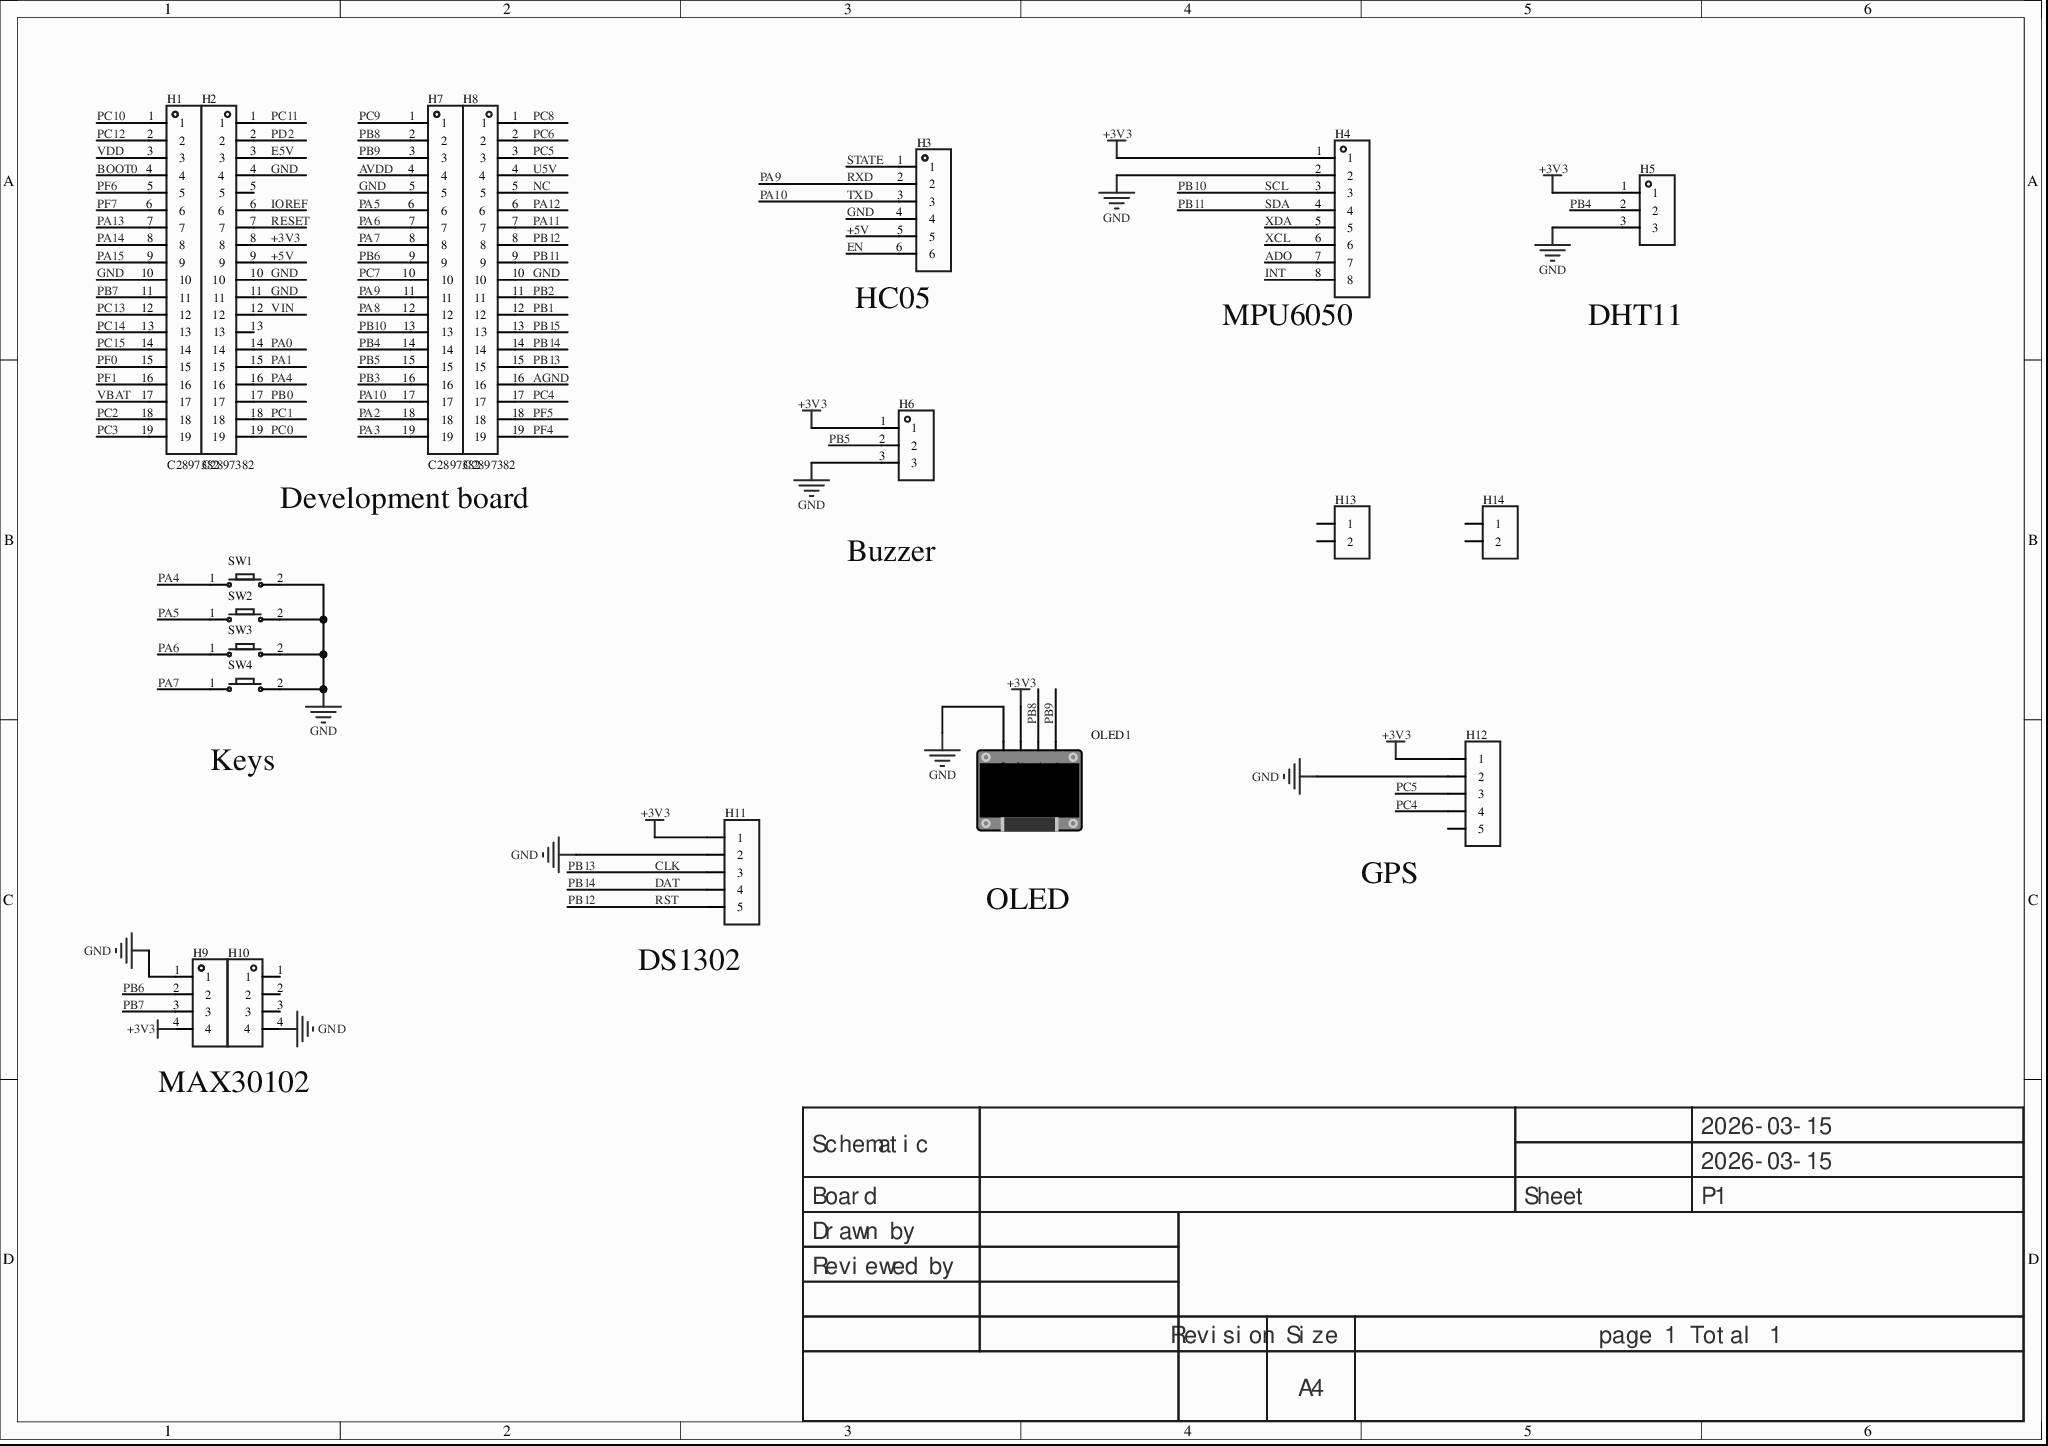
[diagram p0: MISC82907-3.schdoc]
# Altium project MISC82907-2.PrjPcb
1 sheet, 19 parts. Net scope: global (net labels, ports and power ports of the same name join across sheets).
Board file: MISC82907.pcbdoc

## Sheet MISC82907-3.schdoc
size 297 x 209 mm; Version: V1.0; @Project Name: MISC82907; @Update Date: 2026-03-15; @Create Date: 2026-03-15; @Board Name: MISC82907; @Create Time: 16:08:49; @Page Count: 1; @Page No: 1; @Schematic Name: MISC82907; @Update Time: 16:08:49; Size: A4

### Parts
H1  C2897382  [HDR-TH_19P-P2.54-V-F]
H2  C2897382  [HDR-TH_19P-P2.54-V-F]
H3  (no value)  [HDR-TH_6P-P2.54-V-F]
H4  (no value)  [HDR-TH_8P-P2.54-V-F-1]
H5  (no value)  [HDR-TH_3P-P2.54-V-F]
H6  (no value)  [HDR-TH_3P-P2.54-V-F]
H7  C2897382  [HDR-TH_19P-P2.54-V-F]
H8  C2897382  [HDR-TH_19P-P2.54-V-F]
H9  (no value)  [HDR-TH_4P-P2.54-V-F]
H10  (no value)  [HDR-TH_4P-P2.54-V-F]
H11  (no value)  [HDR-TH_5P-P2.54-V-F]
H12  (no value)  [HDR-TH_5P-P2.54-V-F]
H13  (no value)  [HDR-TH_2P-P2.54-V-F]
H14  (no value)  [HDR-TH_2P-P2.54-V-F]
OLED1  (no value)  [0.96OLED_4P]
SW1  (no value)  [Key_SMD_3.6x6.1x2.5]
SW2  (no value)  [Key_SMD_3.6x6.1x2.5]
SW3  (no value)  [Key_SMD_3.6x6.1x2.5]
SW4  (no value)  [Key_SMD_3.6x6.1x2.5]

### Nets
+3V3: H2.8 H4.1 H5.1 H6.1 H9.4 H11.1 H12.1 OLED1.2(VCC)
GND: H1.10 H2.4 H2.10 H2.11 H3.4 H4.2 H5.3 H6.3 H7.5 H8.10 H9.1 H10.4 H11.2 H12.2 OLED1.1(GND) SW1.2 SW2.2 SW3.2 SW4.2
+5V: H2.9 H3.5
ADO: H4.7
AGND: H8.16
AVDD: H7.4
BOOT0: H1.4
CLK: H8.15 H11.3  [also labelled PB13]
DAT: H8.14 H11.4  [also labelled PB14]
E5V: H2.3
EN: H3.6
INT: H4.8
IOREF: H2.6
NC: H8.5
PA0: H2.14
PA1: H2.15
PA2: H7.18
PA3: H7.19
PA4: H2.16 SW1.1
PA5: H7.6 SW2.1
PA6: H7.7 SW3.1
PA7: H7.8 SW4.1
PA8: H7.12
PA9: H3.2 H7.11  [also labelled RXD]
PA10: H3.3 H7.17  [also labelled TXD]
PA11: H8.7
PA12: H8.6
PA13: H1.7
PA14: H1.8
PA15: H1.9
PB0: H2.17
PB1: H8.12
PB2: H8.11
PB3: H7.16
PB4: H5.2 H7.14
PB5: H6.2 H7.15
PB6: H7.9 H9.2
PB7: H1.11 H9.3
PB8: H7.2 OLED1.3(SCL)
PB9: H7.3 OLED1.4(SDA)
PB10: H4.3 H7.13  [also labelled SCL]
PB11: H4.4 H8.9  [also labelled SDA]
PB12: H8.8 H11.5  [also labelled RST]
PB15: H8.13
PC0: H2.19
PC1: H2.18
PC2: H1.18
PC3: H1.19
PC4: H8.17 H12.4
PC5: H8.3 H12.3
PC6: H8.2
PC7: H7.10
PC8: H8.1
PC9: H7.1
PC10: H1.1
PC11: H2.1
PC12: H1.2
PC13: H1.12
PC14: H1.13
PC15: H1.14
PD2: H2.2
PF0: H1.15
PF1: H1.16
PF4: H8.19
PF5: H8.18
PF6: H1.5
PF7: H1.6
RESET: H2.7
STATE: H3.1
U5V: H8.4
VBAT: H1.17
VDD: H1.3
VIN: H2.12
XCL: H4.6
XDA: H4.5

Not connected (* = marked no-connect by the designer): H2 5 13; H10 1 2 3; H12 5; H13 1 2; H14 1 2

### Notes on the sheet
- (near H3) HC05
- (near H4) MPU6050
- DHT11
- Development board
- Buzzer
- (near SW4) Keys
- OLED
- (near H12) GPS
- (near H11) DS1302
- MAX30102
- 2026-03-15
- Schematic
- Board
- Sheet
- P1
- Drawn by
- Reviewed by
- Revision
- Size
- A4
- page 1 Total 1

### Library data of the parts
H1 H2 H7 H8 = HDR-F_2.54_1x19P: ConvertToPcb: yes; ModelId: 131ee080550a465daf9368d356f53fe90819f05c4eef4c71ace90d822a990e87; ModelName: HDR-TH_19P-P2.54-F-LI-1X19P; ModelTransform: 1919.68128,95.6691,0,0,0,0,0,0,-125.984; Symbol: HDR-F_2.54_1x19P; Device: HDR-F_2.54_1x19P; AddInBom: yes; Supplier Footprint: 插件; ManufacturerPart: C2897382; FootprintName: HDR-TH_19P-P2.54-V-F
H3 = HDR-F_2.54_1x6P: Symbol: Header-Female-2.54_1x6; ConvertToPcb: yes; ModelId: 0f5bcf94dcda47d085f24cdca1696fe90819f05c4eef4c71ace90d822a990e87; ModelTransform: 619.684,94.488,0,0,0,0,0,0,-125.984; Device: HDR-F_2.54_1x6P; AddInBom: yes; SupplierPart: C40877; Supplier Footprint: 插件; FootprintName: HDR-TH_6P-P2.54-V-F; ModelName: HDR-TH_6P-P2.54-V-F
H4 = HDR-F_2.54_1x8P: Symbol: Header-Female-2.54_1x8; AddInBom: yes; ModelId: 0f7e4d9227ef4fa08d5469c22cc70cdb0819f05c4eef4c71ace90d822a990e87; ModelName: HDR-F-2.54_1x8; ModelTransform: 799.99844,100,0,0,0,0,0,0,-118.11; Device: HDR-F_2.54_1x8P; ConvertToPcb: yes; FootprintName: HDR-TH_8P-P2.54-V-F-1; SupplierPart: C27438; Supplier Footprint: 插件
H5 H6 = HDR-F_2.54_1x3P: Symbol: PM254V-11-03-H85; ConvertToPcb: yes; ModelId: f3b3cc5aae9641bf9e56fc160cef875b0819f05c4eef4c71ace90d822a990e87; ModelName: HDR2.54-F-LI-1X3P; ModelTransform: 299.9994,100,0,0,0,0,0,0,-118.11; Device: HDR-F_2.54_1x3P; AddInBom: yes; SupplierPart: C541850; Supplier Footprint: 插件; FootprintName: HDR-TH_3P-P2.54-V-F
H9 H10 = HDR-F_2.54_1x4P: Symbol: 2.54-1*4P female; ConvertToPcb: yes; ModelId: d187812051054f85879fcaa51a310d8e0819f05c4eef4c71ace90d822a990e87; ModelTransform: 419.6842,98.464,0,0,0,0,0,0,-118.11; Device: HDR-F_2.54_1x4P; AddInBom: yes; SupplierPart: C2718488; Supplier Footprint: 插件; FootprintName: HDR-TH_4P-P2.54-V-F; ModelName: HDR-TH_4P-P2.54-V-F
H11 = HDR-F_2.54_1x5P: Symbol: Header-Female-2.54_1x5; ConvertToPcb: yes; ModelId: f49cb6116a3d45e5a64915bf3e00773f0819f05c4eef4c71ace90d822a990e87; ModelTransform: 519.684,98.464,0,0,0,0,0,0,-124.016; Device: HDR-F_2.54_1x5P; AddInBom: yes; SupplierPart: C50950; Supplier Footprint: 插件; FootprintName: HDR-TH_5P-P2.54-V-F; ModelName: HDR-TH_5P-P2.54-V-F
H12 = HDR-F_2.54_1x5P: Symbol: Header-Female-2.54_1x5; 3D Model: f49cb6116a3d45e5a64915bf3e00773f0819f05c4eef4c71ace90d822a990e87; 3D Model Transform: 519.684,98.464,0,0,0,0,0,0,-124.016; ConvertToPcb: yes; Device: HDR-F_2.54_1x5P; Supplier Part: C50950; Supplier Footprint: 插件; AddInBom: yes; FootprintName: HDR-TH_5P-P2.54-V-F; ModelName: HDR-TH_5P-P2.54-V-F
H13 H14 = HDR-F_2.54_1x2P: Symbol: Header-Female-2.54_1x2; ConvertToPcb: yes; ModelId: a9450ef445564560a104363b9aacde4e0819f05c4eef4c71ace90d822a990e87; ModelName: HDR-TH_2P-P2.54-F-LI-1X2P; ModelTransform: 215.7476,98.425,0,0,0,0,0,0,-129.921; Device: HDR-F_2.54_1x2P; AddInBom: yes; SupplierPart: C49661; Supplier Footprint: 插件; FootprintName: HDR-TH_2P-P2.54-V-F
OLED1 = 0.96OLED模块_4P: Symbol: 0.96OLED module_4P; ConvertToPcb: yes; ModelId: 79c000fdb68d45a296c2e9bedf4f90550819f05c4eef4c71ace90d822a990e87; ModelTransform: 1393.69792,1318.895,0,0,0,0,0,-560.079,-137.795; Device: 0.96OLED module_4P; AddInBom: yes; FootprintName: 0.96OLED_4P; Supplier Footprint: 插件; ModelName: 0.96OLED_4P
SW1-SW4 = Key_SMD_3.6x6.1x2.5: Symbol: Tactile switch x2; AddInBom: yes; ModelId: 90d18ad19a7e424ebd3215e1b5dcb80c0819f05c4eef4c71ace90d822a990e87; ModelName: KEY-SMD_2P-L6.0-W3.6-H2.5-LS8.0 COPY; ModelTransform: 311.02,141.73,102.36,0,0,0,0,0,0; Device: Key_SMD_3.6x6.1x2.5; ConvertToPcb: yes; FootprintName: Key_SMD_3.6x6.1x2.5; Supplier Footprint: SMD